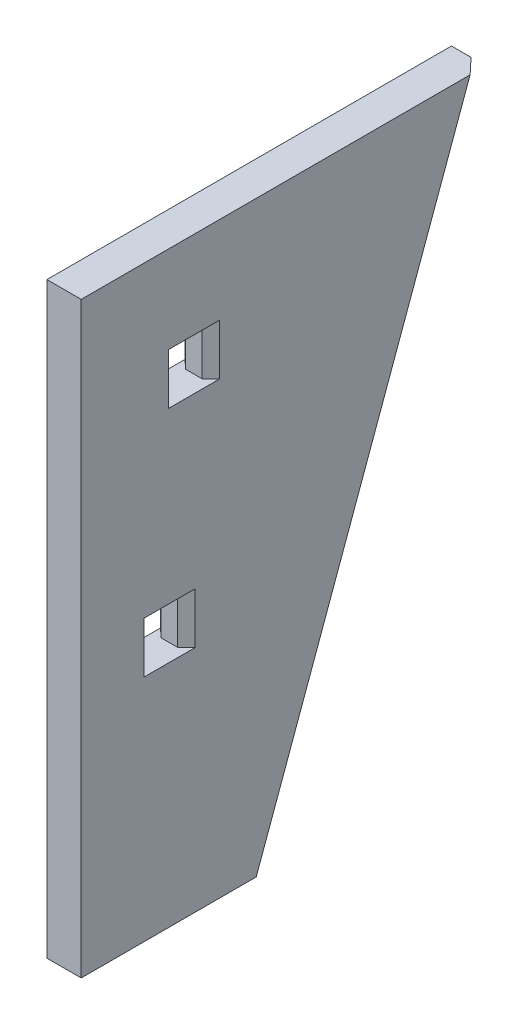
SolidWorks part; units mm, degrees
material "ZG120Mn13-2"
ref_plane "Front Plane" through (0, 0, 0) normal (0, 0, 1) x (1, 0, 0)
ref_plane "Top Plane" through (0, 0, 0) normal (0, 1, 0) x (1, 0, 0)
ref_plane "Right Plane" through (0, 0, 0) normal (1, 0, 0) x (0, 0, -1)
sketch "Sketch1" plane through (0, 0, 0) normal (1, 0, 0) x (0, 0, -1)
  line L0 (0, 0) -> (0, 300)
  line L1 (0, 300) -> (413, 300)
  line L3 (194.6179, -300) -> (0, -300)
  line L4 (0, -300) -> (0, 0)
  line L5 (413, 300) -> (194.6179, -300)
  line L7 (0, 0) -> (273.4876, 0) construction
  dimension "D1" = 413
  dimension "D2" = 20
  dimension "D6" = 600
extrude "Boss-Extrude1" add sketch "Sketch1" along normal mid plane 35
sketch "Sketch2" plane through (0, 0, 0) normal (0, 1, 0) x (1, 0, 0)
  line L0 (0, 0) -> (0, 459.4565) construction
  line L1 (-17.5, 89) -> (-8.5, 97.5)
  line L2 (-17.5, 413) -> (-17.5, 0) construction
  line L3 (-8.5, 97.5) -> (8.5, 97.5)
  line L4 (8.5, 97.5) -> (17.5, 89)
  line L5 (17.5, 413) -> (17.5, 0) construction
  line L6 (-31.4532, 115) -> (29.3887, 115) construction
  line L7 (17.5, 0) -> (-17.5, 0) construction
  line L8 (8.5, 132.5) -> (17.5, 141)
  line L9 (-8.5, 132.5) -> (8.5, 132.5)
  line L10 (-17.5, 141) -> (-8.5, 132.5)
  line L11 (-17.5, 89) -> (-17.5, 141)
  line L12 (17.5, 89) -> (17.5, 141)
  dimension "D1" = 115
  dimension "D2" = 35
  dimension "D3" = 52
  dimension "D4" = 17
extrude "Cut-Extrude1" cut sketch "Sketch2" against normal mid plane 52 from offset 185
chamfer "Chamfer2" distance 15 angle 45 1 edges at (17.5, 0, -303.8089)
sketch "Sketch3" plane through (0, 0, 0) normal (0, 1, 0) x (1, 0, 0)
  line L0 (-45.7619, 90) -> (40.8713, 90) construction
  line L1 (17.5, 0) -> (-17.5, 0) construction
  line L2 (-17.5, 64) -> (-8.5, 72.5)
  line L3 (-17.5, 413) -> (-17.5, 0) construction
  line L4 (-8.5, 72.5) -> (8.5, 72.5)
  line L5 (8.5, 72.5) -> (17.5, 64)
  line L6 (17.5, 397.0373) -> (17.5, 0) construction
  line L7 (0, 0) -> (0, 119.8039) construction
  line L8 (-17.5, 116) -> (-8.5, 107.5)
  line L9 (8.5, 107.5) -> (17.5, 116)
  line L10 (-8.5, 107.5) -> (8.5, 107.5)
  line L11 (-17.5, 64) -> (-17.5, 116)
  line L12 (17.5, 64) -> (17.5, 116)
  dimension "D1" = 90
  dimension "D2" = 35
  dimension "D3" = 52
  dimension "D4" = 17
extrude "Cut-Extrude2" cut sketch "Sketch3" against normal mid plane 52 from offset 40
